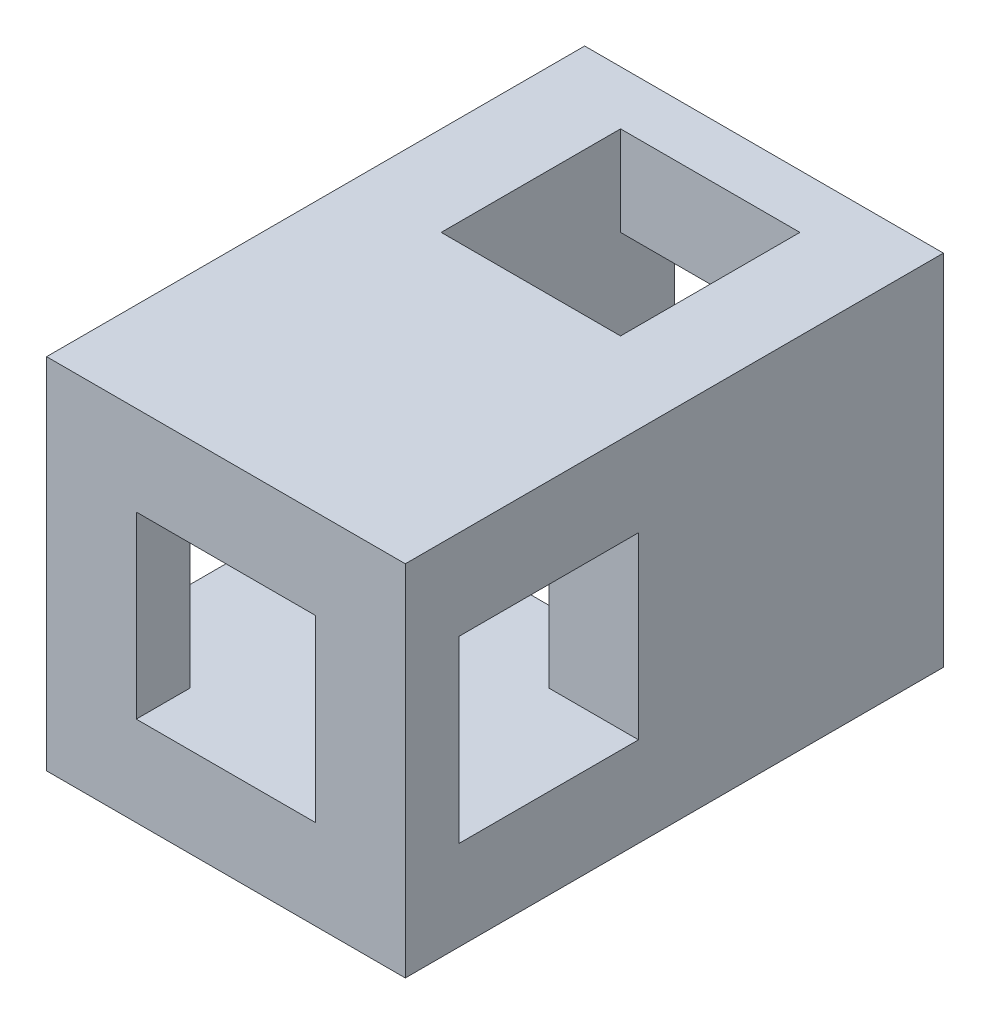
SolidWorks part; units mm, degrees
ref_plane "Front Plane" through (0, 0, 0) normal (0, 0, 1) x (1, 0, 0)
ref_plane "Top Plane" through (0, 0, 0) normal (0, 1, 0) x (1, 0, 0)
ref_plane "Right Plane" through (0, 0, 0) normal (1, 0, 0) x (0, 0, -1)
sketch "Sketch1" plane through (0, 0, 0) normal (0, 0, 1) x (1, 0, 0)
  line L1 (-5, 5) -> (5, 5)
  line L2 (-5, 5) -> (-5, -5)
  line L3 (-5, -5) -> (5, -5)
  line L4 (5, 5) -> (5, -5)
  line L5 (-2.5, 2.5) -> (2.5, 2.5)
  line L7 (-2.5, 2.5) -> (-2.5, -2.5)
  line L8 (-2.5, -2.5) -> (2.5, -2.5)
  line L9 (2.5, 2.5) -> (2.5, -2.5)
  line L10 (-2.5, 2.5) -> (2.5, -2.5) construction
  line L11 (-2.5, -2.5) -> (2.5, 2.5) construction
  point P0 (0, 0)
  point P6 (0, 0)
  dimension "D3" = 5
  dimension "D1" = 10
  dimension "D2" = 10
  dimension "D4" = 5
  dimension "D5" = 5
  dimension "D6" = 5
extrude "Boss-Extrude1" add sketch "Sketch1" along normal blind 15
sketch "Sketch2" plane through (0, 5, 0) normal (0, 1, 0) x (1, 0, 0)
  line L2 (-2.5, -1.5) -> (2.5, -1.5)
  line L3 (-2.5, -1.5) -> (-2.5, -6.5)
  line L4 (-2.5, -6.5) -> (2.5, -6.5)
  line L5 (2.5, -1.5) -> (2.5, -6.5)
  line L6 (-2.5, -1.5) -> (2.5, -6.5) construction
  line L7 (-2.5, -6.5) -> (2.5, -1.5) construction
  line L9 (5, -15) -> (5, 0) construction
  point P0 (0, -4)
  dimension "D1" = 4
  dimension "D3" = 5
  dimension "D2" = 5
  dimension "D4" = 5
extrude "Cut-Extrude1" cut sketch "Sketch2" against normal through all
sketch "Sketch3" plane through (5, 0, 0) normal (1, 0, 0) x (0, 0, -1)
  line L3 (-13.5, 2.5) -> (-8.5, 2.5)
  line L4 (-13.5, 2.5) -> (-13.5, -2.5)
  line L5 (-13.5, -2.5) -> (-8.5, -2.5)
  line L6 (-8.5, 2.5) -> (-8.5, -2.5)
  line L7 (-13.5, 2.5) -> (-8.5, -2.5) construction
  line L8 (-13.5, -2.5) -> (-8.5, 2.5) construction
  line L9 (-15, -5) -> (-15, 5) construction
  line L10 (-15, 5) -> (0, 5) construction
  point P0 (-11, 0)
  dimension "D1" = 4
  dimension "D2" = 5
  dimension "D3" = 5
  dimension "D4" = 5
extrude "Cut-Extrude2" cut sketch "Sketch3" against normal through all
